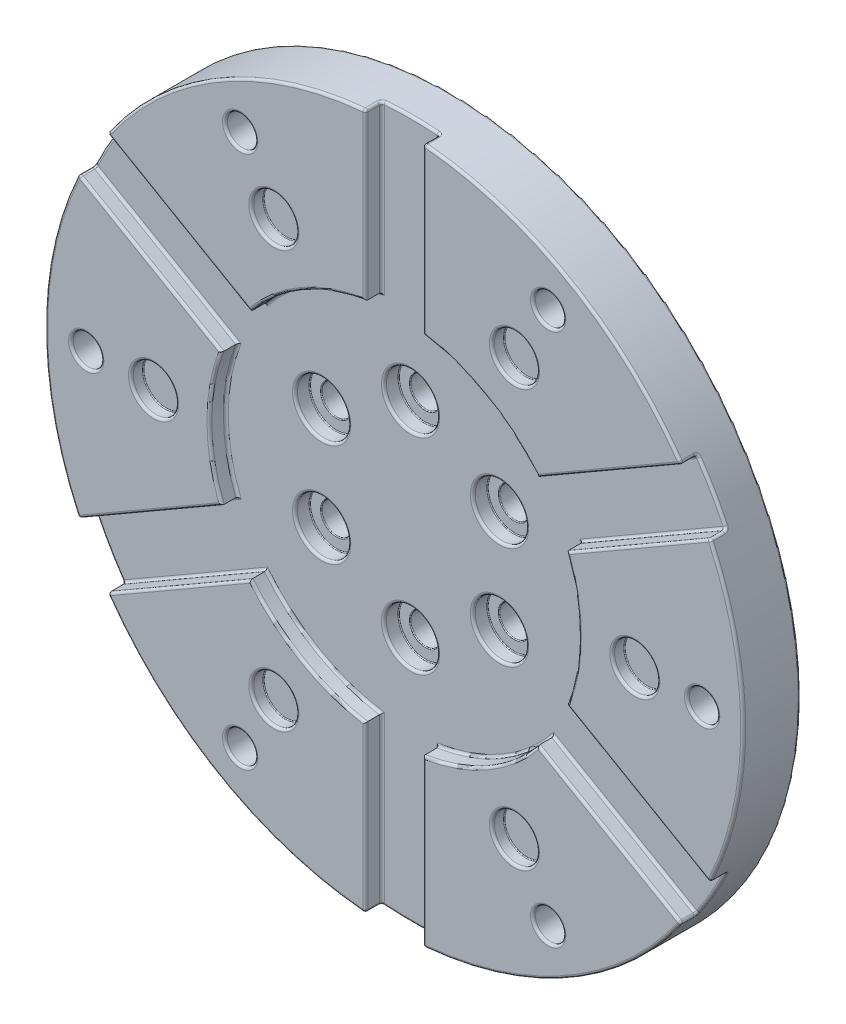
from build123d import *

# Parameters (mm, degrees)
SKETCH1_R           = 42.5
BOSS_EXTRUDE1_DEPTH = 7
SKETCH2_R           = 16.4
BOSS_EXTRUDE2_DEPTH = 5.3
SKETCH3_R           = 1.85
CUT_EXTRUDE4_DEPTH  = 62.349735126
CUT_EXTRUDE8_REACH  = 63.35
SKETCH4_R           = 1.85
CUT_EXTRUDE9_DEPTH  = 2
SKETCH7_R           = 3.25
CUT_EXTRUDE10_DEPTH = 1.8
SKETCH8_R           = 2.75
CUT_EXTRUDE11_DEPTH = 1.5
CUT_EXTRUDE12_DEPTH = 2.5
FILLET2_R           = 0.3
FILLET3_R           = 0.1


with BuildPart() as part:
    # Sketch1 → Boss-Extrude1 (new body)
    with BuildSketch(Plane.XY):
        Circle(SKETCH1_R)
    extrude(amount=BOSS_EXTRUDE1_DEPTH)

    # Sketch2 → Boss-Extrude2 (add)
    with BuildSketch(Plane(origin=(0, 0, 0), x_dir=(-1, 0, 0), z_dir=(0, 0, -1))):
        Circle(SKETCH2_R)
    extrude(amount=BOSS_EXTRUDE2_DEPTH)

    # Sketch3 → Cut-Extrude4 (cut, through all)
    with BuildSketch(Plane(origin=(0, 0, -5.3), x_dir=(-1, 0, 0), z_dir=(0, 0, -1))):
        with Locations((0, 12.5)):
            Circle(SKETCH3_R)
        with Locations((10.825317547, 6.25)):
            Circle(SKETCH3_R)
        with Locations((10.825317547, -6.25)):
            Circle(SKETCH3_R)
        with Locations((0, -12.5)):
            Circle(SKETCH3_R)
        with Locations((-10.825317547, -6.25)):
            Circle(SKETCH3_R)
        with Locations((-10.825317547, 6.25)):
            Circle(SKETCH3_R)
    extrude(amount=-CUT_EXTRUDE4_DEPTH, mode=Mode.SUBTRACT)

    # Sketch4 → Cut-Extrude8 (cut, up to next)
    with BuildSketch(Plane.XY.offset(7), mode=Mode.PRIVATE) as cut_extrude8_sk1:
        with Locations((-37.5, 0)):
            Circle(SKETCH4_R)
    cut_extrude8_tool1 = extrude(cut_extrude8_sk1.sketch, amount=-CUT_EXTRUDE8_REACH, mode=Mode.PRIVATE) & part.part
    # Sketch4 → Cut-Extrude8 (cut, up to next)
    with BuildSketch(Plane.XY.offset(7), mode=Mode.PRIVATE) as cut_extrude8_sk2:
        with Locations((-18.75, 32.475952642)):
            Circle(SKETCH4_R)
    cut_extrude8_tool2 = extrude(cut_extrude8_sk2.sketch, amount=-CUT_EXTRUDE8_REACH, mode=Mode.PRIVATE) & part.part
    # Sketch4 → Cut-Extrude8 (cut, up to next)
    with BuildSketch(Plane.XY.offset(7), mode=Mode.PRIVATE) as cut_extrude8_sk3:
        with Locations((18.75, 32.475952642)):
            Circle(SKETCH4_R)
    cut_extrude8_tool3 = extrude(cut_extrude8_sk3.sketch, amount=-CUT_EXTRUDE8_REACH, mode=Mode.PRIVATE) & part.part
    # Sketch4 → Cut-Extrude8 (cut, up to next)
    with BuildSketch(Plane.XY.offset(7), mode=Mode.PRIVATE) as cut_extrude8_sk4:
        with Locations((37.5, 0)):
            Circle(SKETCH4_R)
    cut_extrude8_tool4 = extrude(cut_extrude8_sk4.sketch, amount=-CUT_EXTRUDE8_REACH, mode=Mode.PRIVATE) & part.part
    # Sketch4 → Cut-Extrude8 (cut, up to next)
    with BuildSketch(Plane.XY.offset(7), mode=Mode.PRIVATE) as cut_extrude8_sk5:
        with Locations((18.75, -32.475952642)):
            Circle(SKETCH4_R)
    cut_extrude8_tool5 = extrude(cut_extrude8_sk5.sketch, amount=-CUT_EXTRUDE8_REACH, mode=Mode.PRIVATE) & part.part
    # Sketch4 → Cut-Extrude8 (cut, up to next)
    with BuildSketch(Plane.XY.offset(7), mode=Mode.PRIVATE) as cut_extrude8_sk6:
        with Locations((-18.75, -32.475952642)):
            Circle(SKETCH4_R)
    cut_extrude8_tool6 = extrude(cut_extrude8_sk6.sketch, amount=-CUT_EXTRUDE8_REACH, mode=Mode.PRIVATE) & part.part
    add(cut_extrude8_tool1.solids().sort_by_distance((-37.5, 0, 7))[0], mode=Mode.SUBTRACT)
    add(cut_extrude8_tool2.solids().sort_by_distance((-18.75, 32.475953, 7))[0], mode=Mode.SUBTRACT)
    add(cut_extrude8_tool3.solids().sort_by_distance((18.75, 32.475953, 7))[0], mode=Mode.SUBTRACT)
    add(cut_extrude8_tool4.solids().sort_by_distance((37.5, 0, 7))[0], mode=Mode.SUBTRACT)
    add(cut_extrude8_tool5.solids().sort_by_distance((18.75, -32.475953, 7))[0], mode=Mode.SUBTRACT)
    add(cut_extrude8_tool6.solids().sort_by_distance((-18.75, -32.475953, 7))[0], mode=Mode.SUBTRACT)

    # Sketch6 → Cut-Extrude9 (cut)
    with BuildSketch(Plane.XY.offset(7)):
        with BuildLine():
            Line((-3.5, 44.470562652), (3.5, 44.470562652))
            Line((3.5, 44.470562652), (3.5, 22.226110771))
            ThreePointArc((3.5, 22.226110771), (11.25, 19.485571585), (17.498376555, 14.144144299))
            Line((17.498376555, 14.144144299), (36.762636977, 25.266370239))
            Line((36.762636977, 25.266370239), (40.262636977, 19.204192413))
            Line((40.262636977, 19.204192413), (20.998376555, 8.081966472))
            ThreePointArc((20.998376555, 8.081966472), (22.5, 0), (20.998376555, -8.081966472))
            Line((20.998376555, -8.081966472), (40.262636977, -19.204192413))
            Line((40.262636977, -19.204192413), (36.762636977, -25.266370239))
            Line((36.762636977, -25.266370239), (17.498376555, -14.144144299))
            ThreePointArc((17.498376555, -14.144144299), (11.25, -19.485571585), (3.5, -22.226110771))
            Line((3.5, -22.226110771), (3.5, -44.470562652))
            Line((3.5, -44.470562652), (-3.5, -44.470562652))
            Line((-3.5, -44.470562652), (-3.5, -22.226110771))
            ThreePointArc((-3.5, -22.226110771), (-11.25, -19.485571585), (-17.498376555, -14.144144299))
            Line((-17.498376555, -14.144144299), (-36.762636977, -25.266370239))
            Line((-36.762636977, -25.266370239), (-40.262636977, -19.204192413))
            Line((-40.262636977, -19.204192413), (-20.998376555, -8.081966472))
            ThreePointArc((-20.998376555, -8.081966472), (-22.5, 0), (-20.998376555, 8.081966472))
            Line((-20.998376555, 8.081966472), (-40.262636977, 19.204192413))
            Line((-40.262636977, 19.204192413), (-36.762636977, 25.266370239))
            Line((-36.762636977, 25.266370239), (-17.498376555, 14.144144299))
            ThreePointArc((-17.498376555, 14.144144299), (-11.25, 19.485571585), (-3.5, 22.226110771))
            Line((-3.5, 22.226110771), (-3.5, 44.470562652))
        make_face()
    extrude(amount=-CUT_EXTRUDE9_DEPTH, mode=Mode.SUBTRACT)

    # Sketch7 → Cut-Extrude10 (cut)
    with BuildSketch(Plane.XY.offset(5)):
        with Locations((0, 12.5)):
            Circle(SKETCH7_R)
        with Locations((10.825317547, 6.25)):
            Circle(SKETCH7_R)
        with Locations((10.825317547, -6.25)):
            Circle(SKETCH7_R)
        with Locations((0, -12.5)):
            Circle(SKETCH7_R)
        with Locations((-10.825317547, -6.25)):
            Circle(SKETCH7_R)
        with Locations((-10.825317547, 6.25)):
            Circle(SKETCH7_R)
    extrude(amount=-CUT_EXTRUDE10_DEPTH, mode=Mode.SUBTRACT)

    # Sketch8 → Cut-Extrude11 (cut)
    with BuildSketch(Plane.XY.offset(7)):
        with Locations((-14.65, 25.374544331)):
            Circle(SKETCH8_R)
        with Locations((14.65, 25.374544331)):
            Circle(SKETCH8_R)
        with Locations((29.3, 0)):
            Circle(SKETCH8_R)
        with Locations((14.65, -25.374544331)):
            Circle(SKETCH8_R)
        with Locations((-14.65, -25.374544331)):
            Circle(SKETCH8_R)
        with Locations((-29.3, 0)):
            Circle(SKETCH8_R)
    extrude(amount=-CUT_EXTRUDE11_DEPTH, mode=Mode.SUBTRACT)

    # Sketch11 → Cut-Extrude12 (cut)
    with BuildSketch(Plane(origin=(0, 0, 0), x_dir=(-1, 0, 0), z_dir=(0, 0, -1))):
        Polygon((18.75, 28.875952642), (21.867691454, 30.675952642), (21.867691454, 34.275952642), (18.75, 36.075952642), (15.632308546, 34.275952642), (15.632308546, 30.675952642), align=None)
        Polygon((-15.632308546, 30.675952642), (-15.632308546, 34.275952642), (-18.75, 36.075952642), (-21.867691454, 34.275952642), (-21.867691454, 30.675952642), (-18.75, 28.875952642), align=None)
        Polygon((34.382308546, -1.8), (37.5, -3.6), (40.617691454, -1.8), (40.617691454, 1.8), (37.5, 3.6), (34.382308546, 1.8), align=None)
        Polygon((15.632308546, -30.675952642), (15.632308546, -34.275952642), (18.75, -36.075952642), (21.867691454, -34.275952642), (21.867691454, -30.675952642), (18.75, -28.875952642), align=None)
        Polygon((-18.75, -28.875952642), (-21.867691454, -30.675952642), (-21.867691454, -34.275952642), (-18.75, -36.075952642), (-15.632308546, -34.275952642), (-15.632308546, -30.675952642), align=None)
        Polygon((-34.382308546, 1.8), (-37.5, 3.6), (-40.617691454, 1.8), (-40.617691454, -1.8), (-37.5, -3.6), (-34.382308546, -1.8), align=None)
    extrude(amount=-CUT_EXTRUDE12_DEPTH, mode=Mode.SUBTRACT)

    # Fillet2
    fillet2_edges = [part.edges().sort_by_distance(p)[0] for p in [
        (-26.214717168, -19.176525898, 7),
        (-11.25, -19.485571585, 7),
        (-3.5, -32.29087397, 7),
        (3.5, -32.29087397, 7),
        (11.25, -19.485571585, 7),
        (26.214717168, -19.176525898, 7),
        (29.714717168, -13.114348072, 7),
        (22.5, 0, 7),
        (22.5, 0, 5),
        (11.25, -19.485571585, 5),
        (-11.25, -19.485571585, 5),
        (-22.5, 0, 5),
        (-11.25, 19.485571585, 5),
        (11.25, 19.485571585, 5),
        (7.575317547, 6.25, 5),
        (1.85, 12.5, -5.3),
        (7.575317547, -6.25, 5),
        (-3.25, -12.5, 5),
        (-14.075317547, -6.25, 5),
        (-42.5, 0, 0),
        (-14.075317547, 6.25, 5),
        (-3.25, 12.5, 5),
        (12.675317547, 6.25, -5.3),
        (-32.05, 0, 7),
        (-17.4, -25.374544331, 7),
        (11.9, -25.374544331, 7),
        (12.675317547, -6.25, -5.3),
        (26.55, 0, 7),
        (11.9, 25.374544331, 7),
        (-17.4, 25.374544331, 7),
        (1.85, -12.5, -5.3),
        (-8.975317547, -6.25, -5.3),
        (34.382308546, 0, 0),
        (35.941154273, 2.7, 0),
        (39.058845727, 2.7, 0),
        (40.617691454, 0, 0),
        (39.058845727, -2.7, 0),
        (35.941154273, -2.7, 0),
        (17.191154273, -29.775952642, 0),
        (20.308845727, -29.775952642, 0),
        (21.867691454, -32.475952642, 0),
        (20.308845727, -35.175952642, 0),
        (17.191154273, -35.175952642, 0),
        (15.632308546, -32.475952642, 0),
        (-8.975317547, 6.25, -5.3),
        (-17.191154273, -29.775952642, 0),
        (-15.632308546, -32.475952642, 0),
        (-17.191154273, -35.175952642, 0),
        (-20.308845727, -35.175952642, 0),
        (-21.867691454, -32.475952642, 0),
        (-20.308845727, -29.775952642, 0),
        (-34.382308546, 0, 0),
        (-35.941154273, -2.7, 0),
        (-39.058845727, -2.7, 0),
        (-40.617691454, 0, 0),
        (-39.058845727, 2.7, 0),
        (-35.941154273, 2.7, 0),
        (17.191154273, 29.775952642, 0),
        (15.632308546, 32.475952642, 0),
        (17.191154273, 35.175952642, 0),
        (20.308845727, 35.175952642, 0),
        (21.867691454, 32.475952642, 0),
        (20.308845727, 29.775952642, 0),
        (-17.191154273, 29.775952642, 0),
        (-20.308845727, 29.775952642, 0),
        (-21.867691454, 32.475952642, 0),
        (-20.308845727, 35.175952642, 0),
        (-17.191154273, 35.175952642, 0),
        (-15.632308546, 32.475952642, 0),
        (-39.35, 0, 7),
        (-20.6, -32.475952642, 7),
        (16.9, -32.475952642, 7),
        (35.65, 0, 7),
        (16.9, 32.475952642, 7),
        (-20.6, 32.475952642, 7),
        (16.4, 0, 0),
        (16.4, 0, -5.3),
        (21.25, 36.806079661, 7),
        (-21.25, 36.806079661, 7),
        (-42.5, 0, 7),
        (-21.25, -36.806079661, 7),
        (21.25, -36.806079661, 7),
        (41.470290304, -9.298657007, 7),
        (29.714717168, 13.114348072, 5),
        (38.431057782, 18.146729671, 6),
        (38.431057782, -18.146729671, 6),
        (29.714717168, -13.114348072, 5),
        (26.214717168, -19.176525898, 5),
        (34.931057782, -24.208907498, 6),
        (3.5, -42.355637169, 6),
        (3.5, -32.29087397, 5),
        (-3.5, -32.29087397, 5),
        (-3.5, -42.355637169, 6),
        (-34.931057782, -24.208907498, 6),
        (-26.214717168, -19.176525898, 5),
        (-29.714717168, -13.114348072, 5),
        (-38.431057782, -18.146729671, 6),
        (-38.431057782, 18.146729671, 6),
        (-29.714717168, 13.114348072, 5),
        (-26.214717168, 19.176525898, 5),
        (-34.931057782, 24.208907498, 6),
        (-3.5, 42.355637169, 6),
        (-3.5, 32.29087397, 5),
        (3.5, 32.29087397, 5),
        (3.5, 42.355637169, 6),
        (34.931057782, 24.208907498, 6),
        (26.214717168, 19.176525898, 5),
        (36.806079661, 21.25, 5),
        (0, 42.5, 5),
        (-36.806079661, 21.25, 5),
        (-36.806079661, -21.25, 5),
        (0, -42.5, 5),
        (36.806079661, -21.25, 5),
        (29.714717168, 13.114348072, 7),
        (26.214717168, 19.176525898, 7),
        (11.25, 19.485571585, 7),
        (3.5, 32.29087397, 7),
        (-3.5, 32.29087397, 7),
        (-11.25, 19.485571585, 7),
        (-26.214717168, 19.176525898, 7),
        (-29.714717168, 13.114348072, 7),
        (-22.5, 0, 7),
        (-29.714717168, -13.114348072, 7),
    ]]
    fillet(fillet2_edges, radius=FILLET2_R)

    # Fillet3
    fillet3_edges = [part.edges().sort_by_distance(p)[0] for p in [
        (7.575317547, 6.25, 3.2),
        (12.675317547, 6.25, 3.2),
        (7.575317547, -6.25, 3.2),
        (12.675317547, -6.25, 3.2),
        (-3.25, -12.5, 3.2),
        (1.85, -12.5, 3.2),
        (-14.075317547, -6.25, 3.2),
        (-8.975317547, -6.25, 3.2),
        (-14.075317547, 6.25, 3.2),
        (-8.975317547, 6.25, 3.2),
        (-3.25, 12.5, 3.2),
        (1.85, 12.5, 3.2),
        (-32.05, 0, 5.5),
        (-17.4, -25.374544331, 5.5),
        (11.9, -25.374544331, 5.5),
        (26.55, 0, 5.5),
        (11.9, 25.374544331, 5.5),
        (-17.4, 25.374544331, 5.5),
        (34.382308546, 0, 2.5),
        (35.941154273, -2.7, 2.5),
        (39.058845727, -2.7, 2.5),
        (40.617691454, 0, 2.5),
        (39.058845727, 2.7, 2.5),
        (35.941154273, 2.7, 2.5),
        (35.65, 0, 2.5),
        (17.191154273, -29.775952642, 2.5),
        (15.632308546, -32.475952642, 2.5),
        (17.191154273, -35.175952642, 2.5),
        (20.308845727, -35.175952642, 2.5),
        (21.867691454, -32.475952642, 2.5),
        (20.308845727, -29.775952642, 2.5),
        (16.9, -32.475952642, 2.5),
        (-17.191154273, -29.775952642, 2.5),
        (-20.308845727, -29.775952642, 2.5),
        (-21.867691454, -32.475952642, 2.5),
        (-20.308845727, -35.175952642, 2.5),
        (-17.191154273, -35.175952642, 2.5),
        (-15.632308546, -32.475952642, 2.5),
        (-20.6, -32.475952642, 2.5),
        (-34.382308546, 0, 2.5),
        (-35.941154273, 2.7, 2.5),
        (-39.058845727, 2.7, 2.5),
        (-40.617691454, 0, 2.5),
        (-39.058845727, -2.7, 2.5),
        (-35.941154273, -2.7, 2.5),
        (-39.35, 0, 2.5),
        (17.191154273, 29.775952642, 2.5),
        (20.308845727, 29.775952642, 2.5),
        (21.867691454, 32.475952642, 2.5),
        (20.308845727, 35.175952642, 2.5),
        (17.191154273, 35.175952642, 2.5),
        (15.632308546, 32.475952642, 2.5),
        (16.9, 32.475952642, 2.5),
        (-17.191154273, 29.775952642, 2.5),
        (-15.632308546, 32.475952642, 2.5),
        (-17.191154273, 35.175952642, 2.5),
        (-20.308845727, 35.175952642, 2.5),
        (-21.867691454, 32.475952642, 2.5),
        (-20.308845727, 29.775952642, 2.5),
        (-20.6, 32.475952642, 2.5),
    ]]
    fillet(fillet3_edges, radius=FILLET3_R)


solid = part.part
